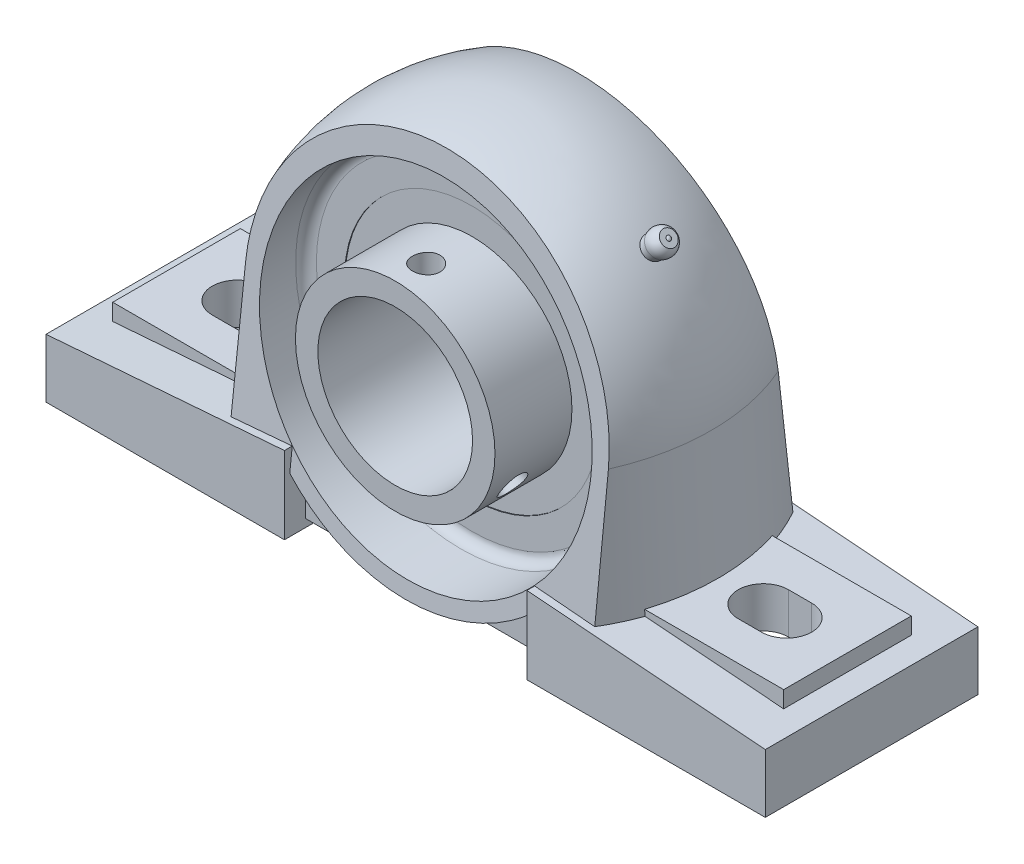
from build123d import *

# Parameters (mm, degrees)
BOSS_EXTRUDE_DEPTH              = 122.2
CUT_EXTRUDE1_DEPTH              = 80.400476324
CUT_EXTRUDE1_DEPTH_BACK         = 80.400476324
SKETCH5_OUTSIDE_W               = 85.446
SKETCH5_OUTSIDE_H               = 131.996
BOSS_EXTRUDE4_REACH             = 81.4
BOSS_EXTRUDE4_DIRECTION_2_REACH = 81.4
BOSS_EXTRUDE1_DEPTH             = 27.5
BOSS_EXTRUDE1_DEPTH_BACK        = 27.5
BOSS_EXTRUDE2_DEPTH             = 16.5
BOSS_EXTRUDE2_DEPTH_BACK        = 16.5
CUT_EXTRUDE3_DEPTH              = 140.878125682
CUT_EXTRUDE4_DEPTH              = 9.4
CUT_EXTRUDE4_DRAFT              = -1
CUT_EXTRUDE4_PROFILE_2_DEPTH    = 9.4
CUT_EXTRUDE4_PROFILE_2_DRAFT    = -1
CIRPATTERN1_COUNT               = 15
SKETCH14_W                      = 49.2
SKETCH14_H                      = 5.8
SKETCH16_W                      = 3.567
SKETCH16_H                      = 8
SKETCH15_W                      = 0.1
SKETCH15_H                      = 7.42
CIRPATTERN2_COUNT               = 2
CIRPATTERN2_ANGLE               = 120


with BuildPart() as part:
    # Sketch1 → Boss-Extrude (new body)
    with BuildSketch(Plane(origin=(0, -47.2, 0), x_dir=(-1, 0, 0), z_dir=(0, 1, 0))):
        with BuildLine():
            Line((-47.716290457, 26.125), (47.716290457, 26.125))
            ThreePointArc((47.716290457, 26.125), (54.4, 0), (47.716290457, -26.125))
            Line((47.716290457, -26.125), (-47.716290457, -26.125))
            ThreePointArc((-47.716290457, -26.125), (-54.4, 0), (-47.716290457, 26.125))
        make_face()
    extrude(amount=BOSS_EXTRUDE_DEPTH)

    # Cut-Sweep1: sweep along a path in Sketch3
    with BuildLine(Plane.XY) as cut_sweep1_path:
        Line((-54.4, -47.2), (-51.514864415, 2.96289458))
        ThreePointArc((-51.514864415, 2.96289458), (0, 51.6), (51.514864415, 2.96289458))
        Line((51.514864415, 2.96289458), (54.4, -47.2))
    # Sketch2 → Cut-Sweep1 (sweep, cut)
    with BuildSketch(Plane(origin=(0, -47.2, 0), x_dir=(-1, 0, 0), z_dir=(0, 1, 0))):
        with BuildLine():
            Line((-47.716290457, 26.125), (-176.6, 26.125))
            Line((-176.6, 26.125), (-176.6, -26.125))
            Line((-176.6, -26.125), (-47.716290457, -26.125))
            ThreePointArc((-47.716290457, -26.125), (-54.4, 0), (-47.716290457, 26.125))
        make_face()
    sweep(path=cut_sweep1_path.line, mode=Mode.SUBTRACT)

    # Sketch5 outside → Cut-Extrude1 (cut, two sides: drawn at the far end of the back side and taken through both)
    with BuildSketch(Plane(origin=(0, 0, 0), x_dir=(0, 0, -1), z_dir=(1, 0, 0)).offset(-CUT_EXTRUDE1_DEPTH_BACK)):
        with Locations((0, 2.2)):
            Rectangle(SKETCH5_OUTSIDE_W, SKETCH5_OUTSIDE_H)
        Polygon((16.5, 52.6), (26.125, -35), (22, -35), (22, -50.2), (-22, -50.2), (-22, -35), (-26.125, -35), (-16.5, 52.6), align=None, mode=Mode.SUBTRACT)
    extrude(amount=CUT_EXTRUDE1_DEPTH + CUT_EXTRUDE1_DEPTH_BACK, mode=Mode.SUBTRACT)

    # Sketch6 → Cut-Revolve2 (revolve, cut)
    with BuildSketch(Plane(origin=(0, 0, 0), x_dir=(0, 0, -1), z_dir=(1, 0, 0)), mode=Mode.PRIVATE) as cut_revolve2_sk:
        with BuildLine():
            Line((-31.413703787, 42.761904762), (-13.179047619, 42.761904762))
            ThreePointArc((-13.179047619, 42.761904762), (-11.28467488, 41.977229881), (-10.5, 40.082857143))
            Line((-10.5, 40.082857143), (-10.5, 38.597279697))
            ThreePointArc((-10.5, 38.597279697), (-9.185281312, 38.931100771), (-7.86, 39.220152983))
            Line((-7.86, 39.220152983), (-7.86, 42.761904762))
            Line((-7.86, 42.761904762), (-5.22, 42.761904762))
            Line((-5.22, 42.761904762), (-5.22, 39.657932372))
            ThreePointArc((-5.22, 39.657932372), (2.692739502, 39.909261506), (10.5, 38.597279697))
            Line((10.5, 38.597279697), (10.5, 40.082857143))
            ThreePointArc((10.5, 40.082857143), (11.28467488, 41.977229881), (13.179047619, 42.761904762))
            Line((13.179047619, 42.761904762), (31.413703787, 42.761904762))
            Line((31.413703787, 42.761904762), (36.112143665, 0))
            Line((36.112143665, 0), (-36.112143665, 0))
            Line((-36.112143665, 0), (-31.413703787, 42.761904762))
        make_face()
    revolve(cut_revolve2_sk.sketch.rotate(Axis((0, 0, 0), (0, 0, -1)), 180), axis=Axis((0, 0, 0), (0, 0, -1)), mode=Mode.SUBTRACT)

    # Sketch11 → Boss-Revolve1 (revolve)
    with BuildSketch(Plane.XY):
        with BuildLine():
            Line((34.192361257, 34.192361257), (40.729350596, 40.729350596))
            ThreePointArc((40.729350596, 40.729350596), (40.447674914, 40.912182849), (40.11596323, 40.964491367))
            Line((40.11596323, 40.964491367), (39.126013736, 41.954440861))
            ThreePointArc((39.126013736, 41.954440861), (37.224951259, 41.609937502), (35.855341314, 40.247260099))
            ThreePointArc((35.855341314, 40.247260099), (35.219120661, 39.234622076), (34.439053677, 38.328140974))
            Line((34.439053677, 38.328140974), (32.247817609, 36.136904906))
            Line((32.247817609, 36.136904906), (34.192361257, 34.192361257))
        make_face()
    revolve(axis=Axis((0, 0, 0), (0.7071067811865476, 0.7071067811865476, 0)))

    # Boss-Extrude4: up to this plane
    boss_extrude4_end = Plane(origin=(-54.4, 52.6, -16.5), z_dir=(0, 0.10921715097101498, -0.9940179142921794))
    # Sketch9 → Boss-Extrude4 (add, up to the surface)
    with BuildSketch(Plane.XY, mode=Mode.PRIVATE) as boss_extrude4_sk1:
        with BuildLine():
            Line((24.567875343, -35), (31.341433126, -35))
            ThreePointArc((31.341433126, -35), (0, -46.981756357), (-31.341433126, -35))
            Line((-31.341433126, -35), (-24.567875343, -35))
            ThreePointArc((-24.567875343, -35), (0, -42.761904762), (24.567875343, -35))
        make_face()
    boss_extrude4_tool1 = split(extrude(boss_extrude4_sk1.sketch, amount=-BOSS_EXTRUDE4_REACH, mode=Mode.PRIVATE), bisect_by=boss_extrude4_end, keep=Keep.BOTH, mode=Mode.PRIVATE)
    add(boss_extrude4_tool1.solids().sort_by_distance((27.954654, -35.638177, 0))[0])

    # Boss-Extrude4 direction 2: up to this plane
    boss_extrude4_direction_2_end = Plane(origin=(-54.4, 52.6, 16.5), z_dir=(0, 0.10921715097101498, 0.9940179142921794))
    # Sketch9 → Boss-Extrude4 direction 2 (add, up to the surface)
    with BuildSketch(Plane.XY, mode=Mode.PRIVATE) as boss_extrude4_direction_2_sk1:
        with BuildLine():
            Line((24.567875343, -35), (31.341433126, -35))
            ThreePointArc((31.341433126, -35), (0, -46.981756357), (-31.341433126, -35))
            Line((-31.341433126, -35), (-24.567875343, -35))
            ThreePointArc((-24.567875343, -35), (0, -42.761904762), (24.567875343, -35))
        make_face()
    boss_extrude4_direction_2_tool1 = split(extrude(boss_extrude4_direction_2_sk1.sketch, amount=BOSS_EXTRUDE4_DIRECTION_2_REACH, mode=Mode.PRIVATE), bisect_by=boss_extrude4_direction_2_end, keep=Keep.BOTH, mode=Mode.PRIVATE)
    add(boss_extrude4_direction_2_tool1.solids().sort_by_distance((27.954654, -35.638177, 0))[0])

    # Sketch4 → Boss-Extrude1 (add, two sides: drawn at the far end of the back side and taken through both)
    with BuildSketch(Plane.XY.offset(-BOSS_EXTRUDE1_DEPTH_BACK)):
        Polygon((31.341433126, -29.2), (93, -34), (93, -49.2), (31.341433126, -49.2), align=None)
        Polygon((-93, -34), (-31.341433126, -29.2), (-31.341433126, -49.2), (-93, -49.2), align=None)
    extrude(amount=BOSS_EXTRUDE1_DEPTH + BOSS_EXTRUDE1_DEPTH_BACK)

    # Sketch8 → Boss-Extrude2 (add, two sides: drawn at the far end of the back side and taken through both)
    with BuildSketch(Plane.XY.offset(-BOSS_EXTRUDE2_DEPTH_BACK)):
        Polygon((31.341433126, -29.2), (86.75, -33.513449606), (86.75, -29.2), align=None)
        Polygon((-86.75, -29.2), (-86.75, -33.513449606), (-31.341433126, -29.2), align=None)
    extrude(amount=BOSS_EXTRUDE2_DEPTH + BOSS_EXTRUDE2_DEPTH_BACK)

    # Sketch7 → Cut-Extrude3 (cut, through all)
    with BuildSketch(Plane.XZ.offset(49.2)):
        with BuildLine():
            Line((-65, 6.5), (-71, 6.5))
            ThreePointArc((-71, 6.5), (-77.5, 0), (-71, -6.5))
            Line((-71, -6.5), (-65, -6.5))
            ThreePointArc((-65, -6.5), (-58.5, 0), (-65, 6.5))
        make_face()
        with BuildLine():
            Line((65, -6.5), (71, -6.5))
            ThreePointArc((71, -6.5), (77.5, 0), (71, 6.5))
            Line((71, 6.5), (65, 6.5))
            ThreePointArc((65, 6.5), (58.5, 0), (65, -6.5))
        make_face()
    extrude(amount=-CUT_EXTRUDE3_DEPTH, mode=Mode.SUBTRACT)


with BuildPart() as cut_extrude4_tool:
    # Sketch10 → Cut-Extrude4 (with draft: the straight prism first)
    with BuildSketch(Plane.XZ.offset(49.2)):
        with BuildLine():
            ThreePointArc((71, -14.41), (71.515492065, -13.165492065), (72.76, -12.65))
            Line((72.76, -12.65), (83.815, -12.65))
            ThreePointArc((83.815, -12.65), (85.059507935, -12.134507935), (85.575, -10.89))
            Line((85.575, -10.89), (85.575, 10.89))
            ThreePointArc((85.575, 10.89), (85.059507935, 12.134507935), (83.815, 12.65))
            Line((83.815, 12.65), (72.76, 12.65))
            ThreePointArc((72.76, 12.65), (71.515492065, 13.165492065), (71, 14.41))
            Line((71, 14.41), (71, 18.315))
            ThreePointArc((71, 18.315), (70.484507935, 19.559507935), (69.24, 20.075))
            Line((69.24, 20.075), (40.526433126, 20.075))
            ThreePointArc((40.526433126, 20.075), (39.281925191, 19.559507935), (38.766433126, 18.315))
            Line((38.766433126, 18.315), (38.766433126, -18.315))
            ThreePointArc((38.766433126, -18.315), (39.281925191, -19.559507935), (40.526433126, -20.075))
            Line((40.526433126, -20.075), (69.24, -20.075))
            ThreePointArc((69.24, -20.075), (70.484507935, -19.559507935), (71, -18.315))
            Line((71, -18.315), (71, -14.41))
        make_face()
    extrude(amount=-CUT_EXTRUDE4_DEPTH)
    # Cut-Extrude4: the draft: its side faces are tilted about the plane it starts from
    cut_extrude4_sides = [cut_extrude4_tool.faces().sort_by_distance(p)[0] for p in [
        (71.515492065, -44.5, -13.165492065),
        (78.2875, -44.5, -12.65),
        (85.059507935, -44.5, -12.134507935),
        (85.575, -44.5, 0),
        (85.059507935, -44.5, 12.134507935),
        (78.2875, -44.5, 12.65),
        (71.515492065, -44.5, 13.165492065),
        (71, -44.5, 16.3625),
        (70.484507935, -44.5, 19.559507935),
        (54.883216563, -44.5, 20.075),
        (39.281925191, -44.5, 19.559507935),
        (38.766433126, -44.5, 0),
        (39.281925191, -44.5, -19.559507935),
        (54.883216563, -44.5, -20.075),
        (70.484507935, -44.5, -19.559507935),
        (71, -44.5, -16.3625),
    ]]
    draft(cut_extrude4_sides, Plane.XZ.offset(49.2), CUT_EXTRUDE4_DRAFT)


with BuildPart() as part_1:
    add(part.part)

    # Cut-Extrude4: cut by cut_extrude4_tool
    add(cut_extrude4_tool.part, mode=Mode.SUBTRACT)


with BuildPart() as cut_extrude4_profile_2_tool:
    # Sketch10 → Cut-Extrude4 profile 2 (with draft: the straight prism first)
    with BuildSketch(Plane.XZ.offset(49.2)):
        with BuildLine():
            Line((-83.815, -12.65), (-72.76, -12.65))
            ThreePointArc((-72.76, -12.65), (-71.515492065, -13.165492065), (-71, -14.41))
            Line((-71, -14.41), (-71, -18.315))
            ThreePointArc((-71, -18.315), (-70.484507935, -19.559507935), (-69.24, -20.075))
            Line((-69.24, -20.075), (-40.526433126, -20.075))
            ThreePointArc((-40.526433126, -20.075), (-39.281925191, -19.559507935), (-38.766433126, -18.315))
            Line((-38.766433126, -18.315), (-38.766433126, 18.315))
            ThreePointArc((-38.766433126, 18.315), (-39.281925191, 19.559507935), (-40.526433126, 20.075))
            Line((-40.526433126, 20.075), (-69.24, 20.075))
            ThreePointArc((-69.24, 20.075), (-70.484507935, 19.559507935), (-71, 18.315))
            Line((-71, 18.315), (-71, 14.41))
            ThreePointArc((-71, 14.41), (-71.515492065, 13.165492065), (-72.76, 12.65))
            Line((-72.76, 12.65), (-83.815, 12.65))
            ThreePointArc((-83.815, 12.65), (-85.059507935, 12.134507935), (-85.575, 10.89))
            Line((-85.575, 10.89), (-85.575, -10.89))
            ThreePointArc((-85.575, -10.89), (-85.059507935, -12.134507935), (-83.815, -12.65))
        make_face()
    extrude(amount=-CUT_EXTRUDE4_PROFILE_2_DEPTH)
    # Cut-Extrude4 profile 2: the draft: its side faces are tilted about the plane it starts from
    cut_extrude4_profile_2_sides = [cut_extrude4_profile_2_tool.faces().sort_by_distance(p)[0] for p in [
        (-85.059507935, -44.5, 12.134507935),
        (-85.575, -44.5, 0),
        (-85.059507935, -44.5, -12.134507935),
        (-78.2875, -44.5, -12.65),
        (-71.515492065, -44.5, -13.165492065),
        (-71, -44.5, -16.3625),
        (-70.484507935, -44.5, -19.559507935),
        (-54.883216563, -44.5, -20.075),
        (-39.281925191, -44.5, -19.559507935),
        (-38.766433126, -44.5, 0),
        (-39.281925191, -44.5, 19.559507935),
        (-54.883216563, -44.5, 20.075),
        (-70.484507935, -44.5, 19.559507935),
        (-71, -44.5, 16.3625),
        (-71.515492065, -44.5, 13.165492065),
        (-78.2875, -44.5, 12.65),
    ]]
    draft(cut_extrude4_profile_2_sides, Plane.XZ.offset(49.2), CUT_EXTRUDE4_PROFILE_2_DRAFT)


with BuildPart() as part_2:
    add(part_1.part)

    # Cut-Extrude4 profile 2: cut by cut_extrude4_profile_2_tool
    add(cut_extrude4_profile_2_tool.part, mode=Mode.SUBTRACT)

    # Sketch12 → Boss-Revolve3 (revolve)
    with BuildSketch(Plane(origin=(0, 0, 0), x_dir=(0, 0, -1), z_dir=(1, 0, 0)), mode=Mode.PRIVATE) as boss_revolve3_sk:
        with BuildLine():
            Line((10.5, 38.617279697), (10.5, 32.82))
            Line((10.5, 32.82), (-10.5, 32.82))
            Line((-10.5, 32.82), (-10.5, 38.617279697))
            ThreePointArc((-10.5, 38.617279697), (0, 40.02), (10.5, 38.617279697))
        make_face()
    revolve(boss_revolve3_sk.sketch.rotate(Axis((0, 0, 0), (0, 0, -1)), 180), axis=Axis((0, 0, 0), (0, 0, -1)))

    # Sketch13 → Boss-Revolve4 (revolve)
    with BuildSketch(Plane(origin=(0, 0, 0), x_dir=(0, 0, -1), z_dir=(1, 0, 0))):
        with BuildLine():
            Line((0, 35.72), (0, 24.32))
            ThreePointArc((0, 24.32), (5.7, 30.02), (0, 35.72))
        make_face()
    boss_revolve4 = revolve(axis=Axis((0, 0, 0), (0, 1, 0)))

    # CirPattern1: Boss-Revolve4 ×15 about axis
    cirpattern1_axis = Axis((0, 0, 0), (0, 0, 1))
    for i in range(1, CIRPATTERN1_COUNT):
        add(boss_revolve4.rotate(cirpattern1_axis, i * 360 / CIRPATTERN1_COUNT))

    # Sketch14 → Boss-Revolve5 (revolve)
    with BuildSketch(Plane(origin=(0, 0, 0), x_dir=(0, 0, -1), z_dir=(1, 0, 0)), mode=Mode.PRIVATE) as boss_revolve5_sk:
        with Locations((-5.6, 22.9)):
            Rectangle(SKETCH14_W, SKETCH14_H)
    revolve(boss_revolve5_sk.sketch.rotate(Axis((0, 0, 0), (0, 0, -1)), 90), axis=Axis((0, 0, 0), (0, 0, -1)))

    # Sketch16 → Cut-Revolve3 (revolve, cut)
    with BuildSketch(Plane(origin=(0, 0, 0), x_dir=(0, 0, -1), z_dir=(1, 0, 0))):
        with Locations((-23.9835, 22)):
            Rectangle(SKETCH16_W, SKETCH16_H)
    cut_revolve3 = revolve(axis=Axis((0, 26, 22.2), (0, -1, 0)), mode=Mode.SUBTRACT)

    # Sketch15 → Boss-Revolve6 (revolve)
    with BuildSketch(Plane(origin=(0, 0, 0), x_dir=(0, 0, -1), z_dir=(1, 0, 0)), mode=Mode.PRIVATE) as boss_revolve6_sk:
        with Locations((-10.25, 29.31)):
            Rectangle(SKETCH15_W, SKETCH15_H)
        with Locations((10.25, 29.31)):
            Rectangle(SKETCH15_W, SKETCH15_H)
    revolve(boss_revolve6_sk.sketch.rotate(Axis((0, 0, 0), (0, 0, -1)), 90), axis=Axis((0, 0, 0), (0, 0, -1)))

    # CirPattern2: Cut-Revolve3 ×2 about axis
    cirpattern2_axis = Axis((0, 0, -21.702927371), (0, 0, -1))
    for i in range(1, CIRPATTERN2_COUNT):
        add(cut_revolve3.rotate(cirpattern2_axis, i * CIRPATTERN2_ANGLE / (CIRPATTERN2_COUNT - 1)), mode=Mode.SUBTRACT)


solid = part_2.part
